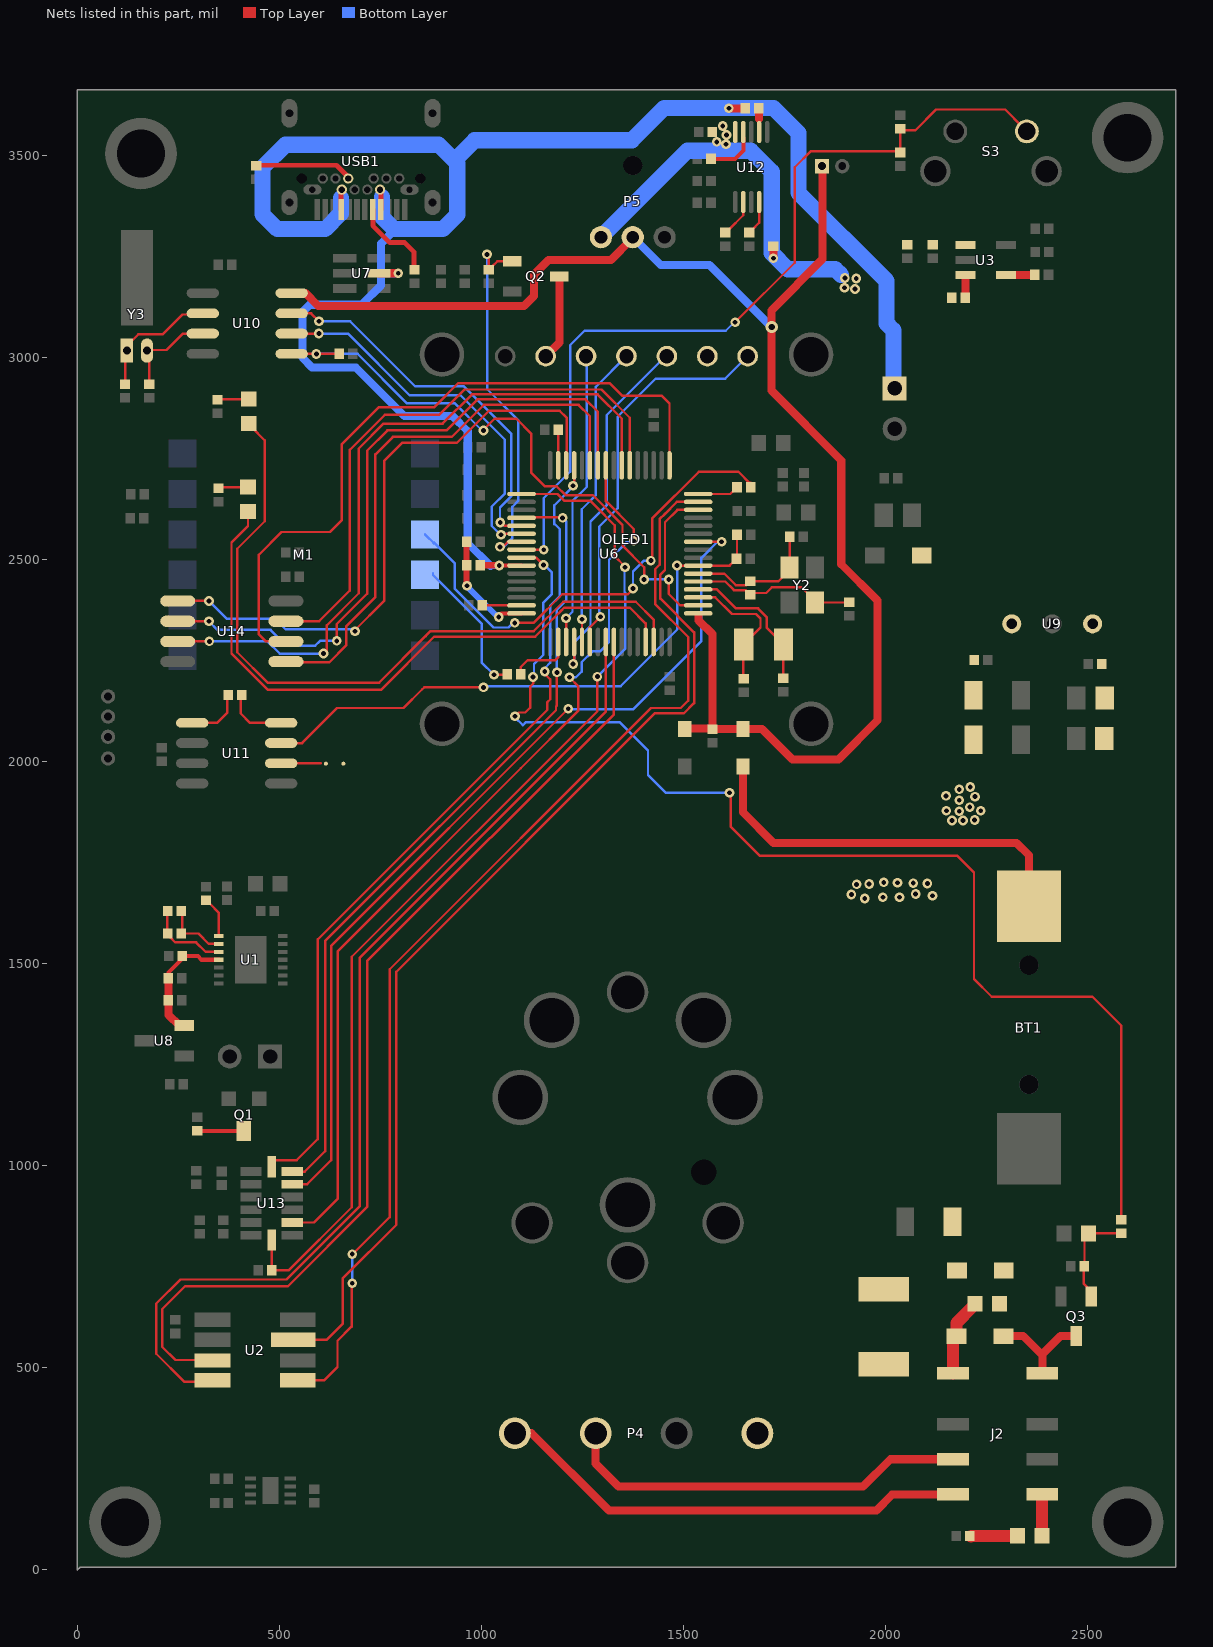
[diagram p0: the nets of this part, all layers, seen from the top]
# Altium PCB MISC105202.PcbDoc (part 3 of 3)
Units mil, origin at the board's own origin, x right, y up, seen from the top; angles counter-clockwise.
Board outline 2717.72 x 3662.2 mil, 4 copper layers (Top Layer, GND, POWER, Bottom Layer), stack 38.217 mil thick; 136 components, 101 nets, 484 pads, 108 vias.
Unrouted connection lines stored in the file: 61.

## Via types
v1: diameter 24, hole 12, Top Layer to Bottom Layer, 107 vias
v2: diameter 30, hole 15, Top Layer to Bottom Layer, 1 vias

## Nets (pads, with @x,y where several pads share a name; then routed paths per layer and width w, separated by ;. In a path a pad name is that pad's centre, name@x,y a point inside that pad or via, vN(x,y) a via of type N, cw(c..) or ccw(c..) an arc to the next point about the centre after c; other vN are vias at no path point) (continued)
INT2: U6.25 U13.9 | length 2323.9
  Top Layer w6: U13.9@531.89,859.45 585.43,859.45 644,918.02 644,1530.22 1097.05,1983.27 1097.22,1983.27 1238.98,2125.03 1238.98,2186.61 v1@1219.68,2205.91 ; U6.25@1307.68,2732.69 1307.68,2644.32 1376.77,2575.24 v1@1376.77,2550.79
  Bottom Layer w6: v1(1217.72,2208.27) 1233.86,2208.27 1247.77,2222.18 1247.77,2245.41 1274.8,2272.44 1292.91,2272.44 1315.35,2294.88 1315.35,2499.21 1358.27,2542.13 1376.77,2542.13 v1(1376.77,2546.06)
K1: C19.1 R24.1 S3.1 U6.40 | length 2150.2
  Top Layer w6: U6.40@1099.02,2524.02 v1(1153.94,2524.02) ; v1@1626.38,3085.43 v1(1627.56,3086.61) 1775,3234.06 1775,3470 1815,3510 C19.1@2036.22,3510 ; C19.1@2038.98,3505.51 2036.22,3508.27 C19.1@2036.22,3510 ; C19.1@2039,3510 C19.1@2036.22,3510 ; S3.1@2338.58,3570.08 2295.67,3612.99 2124.8,3612.99 2073.23,3561.42 2039.96,3561.42 R24.1@2036.22,3565.16 C19.1@2036.22,3510
  Bottom Layer w6: v1(1153.94,2524.02) 1153.94,2651.58 1219.29,2716.93 1219.29,3029.92 1255.12,3065.75 1604.33,3065.75 1625.2,3086.61 v1(1627.56,3086.61)
LCD_PWR: Q2.1 R10.2 U6.39 | length 939.4
  Top Layer w6: v1@1015.75,3253.94 1017.72,3251.97 R10.2@1017.72,3216.73 ; R10.2@1026.38,3224.8 1038.95,3237.37 Q2.1@1076,3237.37 ; v1(1045.59,2531.02) 1052.67,2531.02 1065.36,2543.71 U6.39@1099.02,2543.71
  Bottom Layer w6: v1(1013.78,3254.72) 1014.17,3255.12 1014.17,2920.87 1091.34,2843.7 1091.34,2677.95 1091.34,2645.28 1076.38,2630.31 1076.38,2552.76 1054.64,2531.02 v1(1045.59,2531.02) 1044.01,2531.02 v1@1040.16,2527.17
LED_G: D1.K U6.61 | length 1575.9
  Top Layer w6: D1.K@422.28,2618.27 422.28,2582.52 381.5,2541.73 381.5,2267.5 471.84,2177.17 751.18,2177.17 883.07,2309.06 1117.32,2309.06 1132.82,2309.06 1181.06,2357.29 1181.35,2357.29 1196.33,2372.28 1196.33,2372.56 ; 1196.46,2372.44 1204.33,2380.31 1367.32,2380.31 1406.11,2341.53 U6.61@1406.11,2295.68
LED_R: D2.K U6.62 | length 1890.5
  Top Layer w6: 395.67,2521.65 395.67,2447.63 ; D2.K@431.1,2827.17 463.78,2794.49 463.78,2594.49 395.67,2526.38 395.67,2447.63 ; 861.42,2310.63 872.7,2321.91 1100,2321.91 ; 861.81,2310.24 746.85,2195.28 470.7,2195.28 395.67,2270.3 395.67,2447.63 ; 1100,2322.05 1128.85,2322.05 1202.07,2395.28 1381.5,2395.28 1425.8,2350.98 U6.62@1425.8,2295.68
LMP_C1: C2.2 R4.2 U1.10 | length 197.9
  Top Layer w6: R4.2@222.44,1624.41 222.44,1572.44 229.13,1565.75 229.13,1565.62 242.14,1552.61 293.84,1552.61 317.32,1529.13 U1.10@350.39,1529.13
LMP_C2: C2.1 R4.1 U1.9 | length 149.6
  Top Layer w6: R4.1@259.45,1625.2 259.45,1579.13 264.17,1574.41 299.61,1574.41 325.2,1548.82 U1.9@350.39,1548.82
MR_RST: R26.2 U11.1 | length 149.5
  Top Layer w6: U11.1@284.25,2095.64 346.03,2095.64 370.47,2120.08 R26.2@370.47,2173.23
NetBT1_1: BT1.1 D11.1 | length 942.5
  Top Layer w20: D11.1@1646.85,1987.4 1646.85,1874.41 1722.83,1798.43 2324.02,1798.43 2354.33,1768.11 BT1.1@2354.33,1690.16
NetC8_1: C8.1 U6.4 Y1.1 | length 363.2
  Top Layer w6: U6.4@1536.03,2425.6 1582.67,2425.6 1629.53,2378.74 1684.25,2378.74 1705.51,2357.48 1705.51,2331.5 1746.85,2290.16 C8.1@1746.85,2209.06
NetC22_2: C22.2 R13.2 U6.5 Y2.3 | length 379.5
  Top Layer w6: U6.5@1536.03,2445.28 1603.14,2445.28 1624.41,2424.02 1653.15,2424.02 1660.24,2416.93 1704.33,2416.93 1718.5,2431.1 1790.94,2431.1 1805.91,2416.14 Y2.3@1805.91,2413.78 ; Y2.3@1825.2,2393.31 C22.2@1908.66,2393.31
NetC24_2: C24.2 U6.31 | length 85.2
  Top Layer w6: U6.31@1189.57,2732.69 C24.2@1189.57,2817.92
NetC25_2: C25.2 U6.47 | length 90.6
  Top Layer w6: C25.2@1009.06,2387.8 1010.62,2386.23 U6.47@1099.02,2386.23
NetC26_2: C26.2 R13.1 U6.6 Y2.1 | length 299.2
  Top Layer w6: U6.6@1536.03,2464.97 1600.43,2464.97 1629.38,2436.02 1654.91,2436.02 R13.1@1657.48,2438.58 ; R13.1@1664.96,2445.47 1734.06,2445.47 Y2.1@1750.79,2462.2 ; C26.2@1761.42,2551.57 1762.2,2550.79 Y2.1@1762.2,2479.92
NetC35_2: C35.2 U3.4 | length 67.7
  Top Layer w20: U3.4@2297.45,3203.19 C35.2@2365.19,3203.19
NetC42_2: C42.2 C43.2 C44.1 D4.1 U9.3
NetC48_1: C48.1 U10.2 Y3.1 | length 285.4
  Top Layer w6: C48.1@118.11,2933.27 118.11,3002.76 Y3.1@123.62,3008.27 ; Y3.1@122.44,3016.54 122.44,3028.35 150.79,3056.69 210.63,3056.69 259.84,3105.91 U10.2@286.61,3105.91
NetC49_1: C49.1 U10.3 Y3.2 | length 218.7
  Top Layer w6: Y3.2@174.8,3018.11 220.87,3018.11 261.42,3058.66 U10.3@310.38,3058.66 ; C49.1@178.35,2932.87 Y3.2@178.35,2999.21
NetC53_1: C53.1 U6.3 Y1.2 | length 339
  Top Layer w6: U6.3@1536.03,2405.91 1549.21,2405.91 1578.35,2405.91 1619.29,2364.96 1678.74,2364.96 1690.16,2353.54 1690.16,2331.1 Y1.2@1648.82,2289.76 ; C53.1@1648.03,2207.48 Y1.2@1648.03,2289.76
NetC55_2: C55.2 Q3.1 R31.2 R32.2 | length 229.9
  Top Layer w6: Q3.1@2503.94,693.7 2490.16,707.48 2490.16,750 2491.73,751.57 2491.73,821.65 2502.76,832.68 2502.95,832.48 R32.2@2582.68,832.48
NetD1_A: D1.A R17.1 | length 72.8
  Top Layer w6: R17.1@349.45,2678.9 D1.A@422.28,2678.9
NetD2_A: D2.A R16.1 | length 76.5
  Top Layer w6: R16.1@348.03,2897.64 349.21,2896.46 D2.A@424.02,2896.46
NetD3_1: D3.1 F1.1
NetD5_1: D5.1 J2.8 Q3.3 | length 249.3
  Top Layer w20: D5.1@2304.13,579.13 2339.87,579.13 2388,531 J2.8@2388,490 ; 2388,534 2432.35,578.35 Q3.3@2471.26,578.35 ; J2.8@2393,490 J2.8@2395,492
NetD5_2: D5.2 J2.1 L3.2 | length 180.5
  Top Layer w30: J2.1@2166.7,486.24 D5.2@2166.7,575.7 ; D5.2@2174.93,578 2174.93,610.93 L3.2@2216,652
NetD6_A: D6.A R33.1 | length 119.4
  Top Layer w20: R33.1@2207.73,84 R33.1@2212,84
  Top Layer w30: R33.1@2211,83 2212,84 D6.A@2325.68,84
NetD6_K: D6.K J2.5 | length 100.5
  Top Layer w20: J2.5@2386.31,180.31 J2.5@2386.31,180.69
  Top Layer w30: D6.K@2386.31,84 2386.31,180.31 J2.5@2389,183
NetF1_2: F1.2 P4.1
NetM1_3: M1.3 R7.2 | length 1206.3
  Top Layer w6: v1(1082.28,2342.91) 1128.74,2342.91 1199.61,2413.78 1362.2,2413.78 v1@1376.38,2427.95 ; v1(1418.9,2496.85) 1416.14,2496.85 1422.83,2503.54 1422.83,2601.97 1537.8,2716.93 1635.47,2716.93 R7.2@1665.55,2686.85
  Top Layer w12: R7.2@1665.55,2678.74 R7.2@1665.55,2686.85
  Bottom Layer w6: M1.3@860.24,2561.81 M1.3@882.28,2539.76 ; M1.3@883.46,2540.94 934.25,2490.16 934.25,2427.17 1029.92,2331.5 1066.54,2331.5 1077.95,2342.91 v1(1082.28,2342.91) ; v1(1374.8,2427.95) 1374.8,2469.68 1401.97,2496.85 v1(1418.9,2496.85)
NetM1_4: M1.4 R30.2 | length 352.4
  Top Layer w6: v1(1030.71,2214.57) R30.2@1069.49,2214.57
  Bottom Layer w6: M1.4@879.92,2465.75 879.92,2461.42 1000.39,2340.94 1000.39,2287.4 1000.39,2244.88 v1(1030.71,2214.57)
NetOLED1_2: OLED1.2 Q2.3 | length 204.2
  Top Layer w20: OLED1.2@1158.66,3002.76 1192.52,3036.61 Q2.3@1192.52,3192.91
NetQ1_3: Q1.3 R1.1 | length 112.3
  Top Layer w10: R1.1@297,1086.27 408.27,1086.27 Q1.3@409,1087
NetR3_2: R3.2 U12.9 | length 119
  Top Layer w10: R3.2@1567.73,3491 1627,3491 1648,3512 U12.9@1648,3542
NetR5_1: R5.1 U1.8 | length 90.5
  Top Layer w6: R5.1@326.77,1649.21 350.39,1625.59 U1.8@350.39,1568.5
NetR6_1: R6.1 U12.7 | length 61.8
  Top Layer w6: R6.1@1686.91,3605.91 R6.1@1686.91,3613.29
  Top Layer w10: U12.7@1686.91,3557.35 1686.91,3593 ; R6.1@1686.91,3605.91 R6.1@1687,3606
  Top Layer w20: 1687,3590 R6.1@1687,3608.69
NetR14_1: R14.1 U3.3 | length 56.8
  Top Layer w20: R14.1@2196,3147 2197.45,3148.45 U3.3@2197.45,3203.19
NetR18_1: R18.1 R19.2 U6.48 | length 271.3
  Top Layer w6: R19.2@963.19,2541.14 R19.2@963.39,2541.34
  Top Layer w10: v1@1040.94,2358.66 1048.83,2366.54 U6.48@1099.02,2366.54
  Top Layer w15: v1@963.19,2442.32 R19.2@963.19,2543.7
  Bottom Layer w15: v1@963.58,2434.06 v1@1040.16,2357.48
  other v1: 1042.52,2357.48 964.17,2434.65
NetR22_1: R22.1 USB1.B5 | length 236.9
  Top Layer w12: R22.1@449,3475 641.23,3475 670.28,3445.95 USB1.B5@670.28,3442.38
NetR23_2: R23.2 USB1.A5 | length 207.9
  Top Layer w12: USB1.A5@731.31,3365.69 731.31,3325.78 773.23,3283.86 809.84,3283.86 832.68,3261.02 R23.2@832.68,3221.26
NetR26_1: R26.1 U11.8 | length 161.3
  Top Layer w6: R26.1@403.94,2170.47 403.94,2119.29 427.59,2095.64 U11.8@504.25,2095.64
NetR28_2: R28.2 U12.2 | length 82.8
  Top Layer w6: R28.2@1612,3316 1647.54,3351.54 U12.2@1647.54,3384.12
NetR29_2: R29.2 U12.4 | length 75.1
  Top Layer w6: R29.2@1670,3316 1686.91,3332.91 U12.4@1686.91,3384.12
NetSB1_1: SB1.1 U11.6 | length 72.8
  Top Layer w6: U11.6@529.92,1994.49 530.71,1995.28 602.36,1995.28
NRST: C23.2 R12.1 U6.7 U11.7 | length 1455
  Top Layer w6: U11.7@504.25,2045.64 556.27,2045.64 642.91,2132.28 807.09,2132.28 853.54,2178.74 858.27,2183.46 v1(1004.72,2183.46) ; v1(1483.85,2484.65) U6.7@1536.03,2484.65 1613.79,2484.65 R12.1@1624.41,2495.28 ; R12.1@1632.09,2504.13 C23.2@1632.09,2561.02
  Bottom Layer w6: v1@1005.25,2186.35 1079.96,2186.35 1080.22,2186.61 1344.49,2186.61 1484.39,2326.51 1484.39,2484.12 v1(1483.85,2484.65)
PC13: OLED1.6
PWR: C39.2 C40.2 C41.1 C54.2 D3.2 L3.1 U9.1
  other v1: 1948,1661 1993,1664 2034,1664 2116,1668 1915,1671 2074,1672 1928,1696 1959,1697 2103,1698 2068,1699 2029,1700 1995,1701 2164,1854 2191,1854 2220,1855 2182,1877 2150,1878 2235,1878 2208,1887 2182,1904 2221,1913 2149,1915 2182,1931 2209,1937
QSPI_BK1_IO0: U6.27 U14.5 | length 1366.4
  Top Layer w6: U14.5@533.46,2245.28 623.23,2245.28 664.96,2287.01 664.96,2334.25 737.4,2406.69 737.4,2759.84 780.71,2803.15 926.38,2803.15 1005.51,2882.28 1240.16,2882.28 1268.31,2854.13 U6.27@1268.31,2732.69
QSPI_BK1_IO1: U6.26 U14.2 | length 1696.7
  Top Layer w6: U14.2@248.44,2346.99 v1@326.91,2346.99 ; v1@641.73,2297.24 v1(641.73,2298.43) 641.73,2339.76 716.93,2414.96 716.93,2768.9 767.32,2819.29 913.39,2819.29 989.76,2895.67 1257.48,2895.67 1288,2865.15 U6.26@1288,2732.69
  Bottom Layer w6: v1(325.59,2346.85) 325.2,2346.85 346.46,2325.59 478.35,2325.59 517.32,2286.61 588.58,2286.61 600.39,2298.43 v1(641.73,2298.43)
QSPI_BK1_IO2: U6.23 U14.3 | length 1759.8
  Top Layer w6: U14.3@248.44,2296.99 319.43,2296.99 v1@320.87,2298.43 ; v1(609.06,2266.93) 609.06,2266.14 617.32,2274.41 617.32,2337.01 696.46,2416.14 696.46,2774.41 757.87,2835.83 903.94,2835.83 976.38,2908.27 1287.4,2908.27 1347.06,2848.61 U6.23@1347.06,2732.69
  Bottom Layer w6: v1(326.77,2297.24) 470.47,2297.24 500.79,2266.93 v1(609.06,2266.93)
QSPI_BK1_IO3: U6.22 U14.7 | length 1420.5
  Top Layer w6: U14.7@534.25,2347.24 598.43,2347.24 674.02,2422.83 674.02,2770.87 760.63,2857.48 895.28,2857.48 958.06,2920.27 1297.06,2920.27 1366.74,2850.58 U6.22@1366.74,2732.69
QSPI_BK1_NCS: U6.30 U14.1 | length 1533.9
  Top Layer w6: U14.1@278.35,2398.43 279.53,2397.24 v1(325.59,2397.24) ; v1(687.01,2322.05) 683.86,2322.05 759.06,2397.24 759.06,2743.7 803.54,2788.19 938.58,2788.19 1018.11,2867.72 1193.31,2867.72 1210.38,2850.65 1210.38,2733.8 U6.30@1209.26,2732.69
  Bottom Layer w6: v1(325.59,2397.24) 369.29,2353.54 488.98,2353.54 515.75,2326.77 691.73,2326.77 v1(687.01,2322.05)
QSPI_CLK: U6.17 U14.6 | length 1747.1
  Top Layer w6: U14.6@516.16,2296.99 466.4,2296.99 449.21,2314.17 449.21,2511.42 505.51,2567.72 625.2,2567.72 654.72,2597.24 654.72,2785.43 745.28,2875.98 882.28,2875.98 942.52,2936.22 1316.54,2936.22 1347.64,2905.12 1445.28,2905.12 1465.17,2885.23 U6.17@1465.17,2732.69
R_IN: J2.3 P4.3 | length 1003.3
  Top Layer w20: P4.3@1282,330 1282,263 1339,206 1944,206 2011.65,273.65 J2.3@2166.7,273.65
R_OUT: J2.4 P4.4 | length 1176.7
  Top Layer w20: P4.4@1082.68,338.19 1123.81,338.19 1315,147 1977,147 2016,186 J2.4@2164,186
REF2V5: C37.2 C38.2 R15.1 U1.11 U8.2 | length 291.6
  Top Layer w10: C38.2@225.59,1467.32 225.59,1477.56 266.54,1518.5 298.03,1518.5 307.09,1509.45 U1.11@350.39,1509.45
  Top Layer w20: C37.2@225.2,1409.06 C38.2@225.2,1458.66 ; C37.2@225.98,1409.84 225.98,1373.23 252.76,1346.46 U8.2@264.57,1346.46
Relay: R32.1 U6.41 | length 3033.5
  Top Layer w6: v1(1083.07,2111.81) 1092.39,2121.13 1108.3,2121.13 1120.61,2133.43 1120.61,2185.57 1127.95,2192.91 1127.95,2208.66 v1(1127.56,2209.06) ; U6.41@1099.02,2504.34 1135.03,2504.34 v1(1153.15,2486.22) ; v1(1613.39,1922.83) v1@1614.17,1922.05 ; v1@1616.14,1921.65 1616.14,1839.37 1688.98,1766.54 2177.56,1766.54 2218.5,1725.59 2218.5,1461.81 2262.2,1418.11 2511.42,1418.11 2582.68,1346.85 R32.1@2582.68,865.94
  Bottom Layer w6: v1(1083.07,2111.81) 1083.07,2109.06 1102.36,2089.76 1109.91,2097.31 1341.27,2097.31 1411.81,2026.77 1411.81,1966.54 1455.51,1922.83 v1(1613.39,1922.83) ; v1@1126.38,2207.87 v1(1127.56,2209.06) ; v1@1129.92,2211.42 1129.92,2240.94 1153.15,2264.17 1153.15,2393.31 1174.02,2414.17 1174.02,2467.72 v1@1157.87,2483.86 ; v1@1152.76,2483.86 v1@1153.15,2483.46 ; v1(1153.15,2486.22) v1@1153.15,2483.46 ; v1@1155.31,2481.3 v1@1153.15,2483.46
RTC_CLK: U6.37 U10.7 | length 932.2
  Top Layer w6: U10.7@530.38,3108.66 578.34,3108.66 v1(598,3089) v1@599,3088 ; 1056.29,2583.08 U6.37@1099.02,2583.08
  Bottom Layer w6: v1@601,3089 675,3089 836,2928 956.65,2928 1074.02,2810.63 1074.02,2657.09 1045.67,2628.74 v1@1045.67,2598.43
  other v1: 1046.46,2591.34
RTC_DIO: U6.38 U10.6 | length 940.9
  Top Layer w6: U10.6@530.38,3058.66 v1@591.73,3058.66 ; v1(1048.03,2561.02) v1@1048.03,2563.39 ; v1@1048.02,2563.39 U6.38@1099.02,2563.39
  Bottom Layer w6: v1(597.64,3058.66) 669.34,3058.66 822,2906 947.94,2906 1057.87,2796.06 1057.87,2662.99 1025.46,2630.57 1025.46,2582.64 1045.1,2562.99 v1@1047.64,2562.99
RTC_RST: R25.1 U6.2 U10.5 | length 1465.3
  Top Layer w6: U10.5@530.38,3008.66 v1@585.83,3008.66 ; v1@592.91,3009.45 593.7,3008.66 R25.1@647.83,3008.66 ; v1(1005.12,2818.9) 1005.12,2820.87 1032.68,2848.43 1085.83,2848.43 1122.83,2811.42 1122.83,2715.35 1157.48,2680.71 1186.22,2680.71 1207.87,2659.06 1275.2,2659.06 1348.82,2585.43 1348.82,2534.25 1402.36,2480.71 v1(1402.36,2450.39) ; v1(1463.39,2450.39) 1463.39,2414.57 1491.72,2386.23 U6.2@1536.03,2386.23
  Bottom Layer w6: v1(591.34,3008.27) 693.73,3008.27 816,2886 934.08,2886 1003.15,2816.93 v1(1005.12,2818.9) ; v1(1402.36,2450.39) v1(1463.39,2450.39)
SPI1_MISO: U2.8 U6.56 | length 2544.3
  Top Layer w6: U2.8@334.46,468.9 331.51,465.95 263.97,465.95 195.28,534.65 195.28,658.66 255.12,718.5 517.36,718.5 699,900.14 699,1514.75 1307.68,2123.43 U6.56@1307.68,2295.68
SPI1_MOSI: U2.7 U6.57 | length 2480.9
  Top Layer w6: U2.7@321.65,519.29 242.52,519.29 209.84,551.97 209.84,644.88 266.54,701.57 520.87,701.57 717,897.71 717,1505.98 1327.37,2116.35 U6.57@1327.37,2295.68
SPI1_NCS: U2.3 U6.14 | length 2640.9
  Top Layer w6: U2.3@551.57,568.9 616.54,568.9 656.3,608.66 656.3,720.87 789,853.57 789,1479.55 1428.35,2118.9 1500.39,2118.9 1525.98,2144.49 1525.98,2319.29 1442.39,2402.89 1442.39,2462.59 1453.94,2474.14 1453.94,2591.73 1484.65,2622.45 U6.14@1536.03,2622.45
SPI1_SCK: U2.1 U6.15 | length 2760.7
  Top Layer w6: U2.1@545.48,468.9 610.24,468.9 643.7,502.36 643.7,566.93 678.74,601.97 v1@678.74,706.3 ; v1(680.31,781.1) 681.5,781.1 773,872.61 773,1485.99 1419.29,2132.28 1492.91,2132.28 1511.42,2150.79 1511.42,2307.87 1429.53,2389.76 1429.53,2475.59 1440.55,2486.61 1440.55,2599.61 1453.54,2612.6 1483.08,2642.13 U6.15@1536.03,2642.13
  Bottom Layer w6: v1(680.31,709.06) v1(680.31,781.1)
SPI2_MISO: U6.10 U13.12 | length 2209.3
  Top Layer w6: U13.12@531.89,953.94 568.5,953.94 628,1013.43 628,1543.75 v1(1214.57,2130.31) ; U6.10@1536.03,2543.71 v1(1594.09,2543.71)
  Bottom Layer w6: v1@1215.35,2129.53 1375.59,2129.53 1544.09,2298.03 1544.09,2503.54 1584.26,2543.71 v1(1594.09,2543.71)
SPI2_MOSI: U6.36 U13.13 | length 2024.4
  Top Layer w6: U13.13@531.89,985.43 562.6,985.43 613,1035.83 613,1555.52 1184.25,2126.77 1184.25,2135.83 1186.61,2138.19 v1(1186.61,2220.47) ; U6.36@1099.02,2602.76 1100.34,2604.08 1199.48,2604.08 v1(1200.8,2602.76)
  Bottom Layer w6: v1@1187.01,2220.87 v1(1186.61,2220.47) 1186.61,2376.38 1209.84,2399.61 1209.84,2593.72 v1(1200.8,2602.76) v1@1201.57,2603.54
SPI2_NCS: R11.1 U6.33 U13.7 | length 2584.2
  Top Layer w6: R11.1@480.79,741.65 U13.7@480.79,816.22 ; R11.1@480.91,740.94 522.83,740.94 679,897.11 679,1516.75 1286.61,2124.37 v1(1286.61,2209.84) v1@1286.61,2214.17 ; U6.33@1099.56,2661.28 U6.33@1099.02,2661.82 1187.79,2661.82 1204.93,2644.68 1269.5,2644.68 1281.89,2632.28 ; 1281.69,2632.09 1329.33,2584.45 1329.33,2508.07 v1@1354.33,2483.07 ; v1@1355.77,2483.07 1355.77,2480.45 v1@1355.91,2480.31
  Bottom Layer w6: v1(1286.61,2209.84) 1355.12,2278.35 1355.12,2417.94 1353.8,2419.25 1353.8,2479.39 v1(1355.12,2480.71)
SPI2_SCK: U6.29 U13.14 | length 2114.6
  Top Layer w6: U13.14@480.79,997.17 480.79,1013.46 542.6,1013.46 595,1065.87 595,1559.96 1162.99,2127.95 1162.99,2146.85 1170.08,2153.94 1170.08,2203.15 v1@1155.91,2217.32 ; v1@1228.94,2684.85 U6.29@1228.94,2732.69
  Bottom Layer w6: v1(1156.61,2222.43) 1156.61,2215.27 1156.3,2214.96 1156.3,2230.71 1170.2,2244.61 1170.2,2385.56 1194.09,2409.45 1194.09,2574.41 1181.1,2587.4 ; 1179.8,2587.4 1179.8,2633.73 v1@1224.02,2677.95 ; v1@1224.02,2678.74 v1@1224.02,2677.95 ; v1@1224.8,2683.46 1223.62,2682.28 v1(1226.38,2682.28) ; v1@1226.77,2680.71 v1@1224.02,2677.95
SPI3_MISO: OLED1.5 U6.52 | length 921.2
  Top Layer w6: v1(1226.77,2241.34) 1227.17,2241.34 1229.92,2244.09 1229.92,2239.37 1228.94,2238.39 U6.52@1228.94,2295.68
  Bottom Layer w6: v1@1228.35,2237.8 1228.94,2238.39 1228.94,2294.69 1269.63,2335.38 1269.63,2593.65 1309.45,2633.46 1309.45,2856.69 OLED1.5@1451.57,2998.82
SPI3_MOSI: OLED1.4 U6.53 | length 749.6
  Top Layer w6: U6.53@1248.63,2295.68 v1(1248.63,2351.78)
  Bottom Layer w6: v1@1248.03,2355.12 1248.03,2624.02 1283.07,2659.06 1283.07,2927.17 OLED1.4@1358.66,3002.76
SPI3_NCS: OLED1.7 U6.54 | length 972.5
  Top Layer w6: U6.54@1269.63,2296.99 U6.54@1268.31,2295.68 1268.31,2332.09 1294.88,2358.66 v1@1294.88,2363.39
  Bottom Layer w6: v1@1291.34,2363.78 1291.34,2581.1 1337.01,2626.77 1337.01,2853.15 1430.71,2946.85 1602.76,2946.85 OLED1.7@1658.66,3002.76
  other v1: 1294.09,2358.27
SPI3_SCK: OLED1.3 U6.51 | length 723.4
  Top Layer w6: U6.51@1209.26,2295.68 v1(1209.26,2354.54)
  Bottom Layer w6: v1@1211.42,2356.69 v1(1209.26,2354.54) 1225.2,2370.47 1225.2,2644.09 1260.24,2679.13 OLED1.3@1260.24,2994.88
UART2RX: R30.1 U6.50 | length 155.9
  Top Layer w6: R30.1@1097.24,2219.29 1097.24,2233.46 1114.56,2250.78 1183.07,2250.78 1189.57,2257.29 U6.50@1189.57,2295.68 ; R30.1@1098.03,2215.75 R30.1@1098.03,2216.93
UART2TX: R7.1 U6.16 | length 93.8
  Top Layer w6: U6.16@1536.03,2661.82 1615.36,2661.82 R7.1@1625.59,2672.05
USB_OTGFS_VBUS: J1.1 R6.2 R18.2 U6.42 U7.5 USB1.A4 USB1.A9 USB1.B4 USB1.B9 | length 4621.5
  Top Layer w10: v1@1054.32,2484.65 U6.42@1099.02,2484.65
  Top Layer w12: USB1.A9@652.57,3365.69 USB1.B4@652.57,3413.59 ; USB1.B9@750.79,3415.35 750.99,3415.15 USB1.A4@750.99,3365.69
  Top Layer w15: R18.2@999.61,2484.65 1000.39,2485.43 v1@1044,2485.43
  Top Layer w20: U7.5@746.26,3207.87 v1(794.13,3207.87) ; v1(1612,3616) R6.2@1652.27,3616
  Bottom Layer w15: 1021.85,2484.15 v1@1043.15,2484.15
  Bottom Layer w20: 577,3132 557,3112 557,2999 581,2975 689,2975 809,2855 928,2855 966,2817 966,2540 1021.85,2484.15 ; 579,3130 703,3130 751,3178 751,3281 780,3310 ; 655,3394 USB1.B4@655,3413 ; 751,3396.85 USB1.B9@751,3413 ; 754,3208 v1@793,3208
  Bottom Layer w40: 652,3394 652,3356 613,3317 495,3317 458,3354 458,3469 515,3526 894,3526 940,3480 940,3353 904,3317 784,3317 754.15,3346.85 754.15,3396.85 ; 940,3494 983,3537 1372,3537 1452,3617 1722,3617 1784,3555 1784,3407 2002,3189 2002,3084 2019,3067 J1.1@2019,2933
  other v1: 1044,2485
VBAT: C56.2 D10.2 D11.2 P1.1 P5.2 U6.1 U10.8 | length 3745
  Top Layer w20: U10.8@530.38,3158.66 564.34,3158.66 596,3127 1105,3127 1130,3152 1130,3205 1166,3241 1320,3241 P5.2@1371,3292 ; D10.2@1507.48,2081.1 1568.11,2081.1 1571.26,2084.25 1571.26,2314.96 1537.01,2349.21 1537.01,2358.66 ; C56.2@1571.65,2080.12 D11.2@1639.96,2080.12 ; D11.2@1646.85,2080.31 1693.68,2080.31 1769,2005 1883,2005 1980,2102 1980,2398 1890,2488 1890,2745 1717,2918 1717,3116 1844,3243 P1.1@1844,3470
  Bottom Layer w20: P5.2@1374.23,3297.15 1443.38,3228 1564,3228 1717,3075 v2(1718,3075)
VPACK: C6.1 C16.2 P5.3 R2.2 R14.2 R27.2 U3.1 U12.10 | length 963.7
  Top Layer w10: R2.2@1722,3274.27 R2.2@1728.7,3274.27
  Top Layer w20: v1(1722,3245) R2.2@1722,3274.27
  Bottom Layer w40: P5.3@1295.49,3297.15 1509.34,3511 1666,3511 1718,3459 1718,3258 1758,3218 1875,3218 1889.5,3203.5
  other v1: 1924,3169 1898,3172 1927,3195 1899,3196 1605,3527 1582,3533 1606,3550 1597,3572
WDI: SB1.2
pads on no net: BT1.0 J2.2 J2.7 M1.1 M1.6 M1.7 M1.9 M1.10 M1.12 OLED1.0 P5.0 P5.1 S2.0 S3.0 U1.5 U2.4 U4.3 U5.3 U5.6 U6.28 U6.43 U7.3 U7.4 U11.4 U11.5 U12.6 U13.3 U13.10 USB1.0 USB1.A2 USB1.A3 USB1.A8 USB1.A10 USB1.A11 USB1.B2 USB1.B3 USB1.B8 USB1.B10 USB1.B11 Y2.2 Y2.4 Y3.Y3

## Polygon pours and split planes (outlines as drawn)
VPACK on Top Layer "Top Layer-No Net" (solid, remove dead copper): 2186,3330 1950,3330 1901,3281 1884,3264 1884,3225 1884,3150 1906,3128 1930,3104 1960,3104 2167,3104 2170,3107 2176,3113 2176,3136 2176,3160 2174,3162 2173,3163 2166,3163 2042,3163 2021,3184 2009,3196 2009,3226 2009,3247 2019,3257 2028,3266 2042,3266 2223,3266 2227,3270 2229,3272 2229,3283 2229,3315 2223,3321 2214,3330 2186,3330
VPACK on Top Layer "Top Layer-No Net" (solid, remove dead copper): 1557,3558.19 1557,3531.54 1562.07,3525.75 1573.21,3513 1596.51,3513 1625.89,3513 1630.96,3518.79 1634,3522.27 1634,3532.7 1634,3582.52 1630.96,3586 1603.61,3586 1576.25,3586 1566.12,3574.41 1557,3563.98 1557,3558.19
+5 on Top Layer "Top Layer-No Net" (solid, remove dead copper): 1555,3431 1555,3366 1565,3356 1580,3341 1606,3341 1617,3341 1630,3354 1633,3357 1633,3372 1633,3414 1622,3425 1596,3451 1577,3451 1558,3451 1555,3448 1555,3429
+5 on Top Layer "Top Layer-No Net" (solid, remove dead copper): 1927,2619 1927,2502 1937,2492 1947,2482 1960,2482 1998,2482 2002,2486 2020,2504 2020,2592 2020,2648 2013,2655 2008,2660 2008,2696 2008,2755 2028,2775 2058,2805 2058,2829 2058,2843 2047,2854 2041,2860 2019,2860 1983,2860 1972,2849 1927,2804 1927,2619
NetC42_2 on Top Layer "Top Layer-No Net" (solid, remove dead copper): 2522,2243 2522,2206 2519,2203 2516,2200 2516,2188 2516,2028 2519,2025 2520,2024 2526,2024 2582,2024 2587,2029 2592,2034 2592,2060 2592,2403 2560,2435 2454,2541 2179,2541 2070,2541 2062,2533 2060,2531 2060,2514 2060,2474 2060,2465 2082,2443 2085,2440 2160,2440 2427,2440 2449,2418 2475,2392 2475,2363 2475,2313 2506,2282 2522,2266 2522,2244
PWR on Top Layer "Top Layer-No Net" (solid, remove dead copper): 2135,2224 2135,1855 2139,1851 2153,1837 2159,1837 2225,1837 2233,1845 2249,1861 2249,2184 2249,2207 2241,2215 2230,2226 2230,2240 2230,2272 2237,2279 2259,2301 2291,2301 2322,2301 2330,2309 2340,2319 2340,2333 2340,2371 2333,2378 2329,2382 2296,2382 2232,2382 2204,2354 2135,2285 2135,2225
PWR on Top Layer "Top Layer-No Net" (solid, remove dead copper): 2136,920 2136,819 2145,810 2148,807 2158,807 2235,807 2235,805 2253,787 2262,778 2262,669 2262,638 2264,636 2266,634 2271,634 2334,634 2338,638 2344,644 2344,660 2344,852 2260,936 2236,960 2236,1060 2236,1327 2162,1401 2141,1422 2141,1560 2141,1685 2112,1714 2096,1730 2046,1730 1926,1730 1908,1712 1883,1687 1883,1644 1883,1361 2073,1171 2136,1108 2136,920
NetD3_1 on Top Layer "Top Layer-No Net" (solid, remove dead copper): 1922,721 1922,666 1927,661 1933,655 1945,655 2130,655 2154,679 2172,697 2188,697 2197,697 2207,707 2212,712 2212,736 2212,771 2201,782 2160,782 1960,782 1933,755 1922,744 1922,721
NetF1_2 on Top Layer "Top Layer-No Net" (solid, remove dead copper): 1629,364 1629,314 1629,305 1638,296 1648,286 1670,286 1854,286 1885,317 1915,347 1955,347 2032,347 2051,366 2065,380 2065,473 2065,541 2054,552 2052,554 1933,554 1857,554 1823,520 1745,442 1709,442 1677,442 1662,427 1629,394 1629,364
VPACK on Bottom Layer "Top Layer-No Net" (solid, remove dead copper): 1871,3196 1871,3170 1881,3160 1889,3152 1897,3152 1935,3152 1939,3156 1946,3163 1946,3171 1946,3201 1941,3206 1927,3220 1920,3220 1882,3220 1872,3210 1871,3209 1871,3197
VPACK on Bottom Layer "Top Layer-No Net" (solid, remove dead copper): 1550,3549 1550,3519 1564,3505 1571,3498 1594,3498 1613,3498 1623,3508 1628,3513 1628,3531 1628,3574 1618,3584 1614,3588 1594,3588 1574,3588 1560,3574 1550,3564 1550,3548
+5 on Bottom Layer "Top Layer-No Net" (solid, remove dead copper): 1573,3409 1573,3349 1579,3343 1583,3339 1592,3339 1615,3339 1618,3342 1624,3348 1624,3357 1624,3421 1618,3427 1612,3433 1605,3433 1591,3433 1586,3428 1573,3415 1573,3408
PWR on Bottom Layer "Top Layer-No Net" (solid, remove dead copper): 1896,1715 1896,1653 1908,1641 1917,1632 1940,1632 2117,1632 2148,1663 2264,1779 2264,1862 2264,1919 2244,1939 2232,1951 2231,1952 2127,1952 2091,1952 2028,1889 1896,1757 1896,1714
GND on GND (split plane): 2697.23,26.79 20.09,26.79 19.71,3641.71 2697.23,3641.71
3V3 on POWER (split plane): 2697.23,26.79 20.09,26.79 19.71,3641.71 2697.23,3641.71
USB_OTGFS_VBUS on POWER (split plane): 1312.91,2587.59 1312.91,2359.94 1292.82,2339.85 1161.18,2339.85 1051.13,2449.9 1049.04,2451.5 1046.61,2452.51 1044,2452.85 748,2452.85 745.39,2452.51 742.96,2451.5 740.87,2449.9 692.87,2401.9 691.27,2399.81 690.26,2397.37 689.91,2394.76 689.91,2281.76 690.26,2279.15 691.27,2276.72 692.87,2274.63 809.91,2157.59 809.91,1999.94 680.82,1870.85 595.18,1870.85 587.09,1878.94 587.09,1965.76 586.74,1968.37 585.73,1970.81 584.13,1972.9 531.13,2025.9 529.04,2027.5 526.61,2028.51 524,2028.85 439.18,2028.85 351.13,2116.9 349.04,2118.5 346.61,2119.51 344,2119.85 220.18,2119.85 197.09,2142.94 197.09,2257.76 197.09,2403.59 442.18,2648.68 1251.82,2648.68

## Keep-outs
Keep-Out Layer:
  lines w7.87: 0,0 0,3661.42 2716.54,3661.42 2716.54,0 0,0

## Other copper
POWER (plane layer: these items are gaps in the copper):
  lines w20: 187,2246.76 187,2407.76 438,2658.76 1256,2658.76 1323,2591.76 1323,2355.76 1297,2329.76 1157,2329.76 1044,2442.76 748,2442.76 700,2394.76 700,2281.76 820,2161.76 820,1995.76 685,1860.76 591,1860.76 577,1874.76 577,1965.76 524,2018.76 435,2018.76 344,2109.76 216,2109.76 187,2138.76 187,2257.76

## Silkscreen, mask and mechanical layers (free items; w line width, h text height)
Top Overlay:
  lines w7.87: 0,1771.65 2716.54,1771.65 ; 0,1889.76 2716.52,1897.78
Bottom Overlay:
  text "ShockRecord_B_V0.4" at 1369,1890.76 h35
  text "2017.12" at 7805,1588.76 h90
  text "V0.347" at 7995,1483.76 h90
  text "2018-05-19" at 1658,1461.76 h35